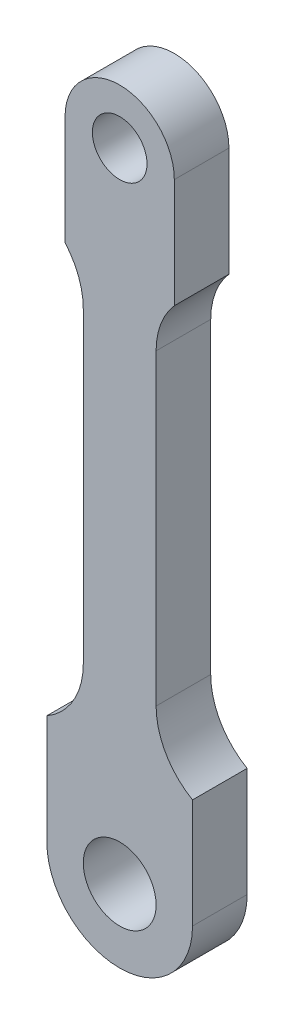
SolidWorks part; units mm, degrees
ref_plane "Front Plane" through (0, 0, 0) normal (0, 0, 1) x (1, 0, 0)
ref_plane "Top Plane" through (0, 0, 0) normal (0, 1, 0) x (1, 0, 0)
ref_plane "Right Plane" through (0, 0, 0) normal (1, 0, 0) x (0, 0, -1)
other "Configuration Table"
sketch "Sketch1" plane through (0, 0, 0) normal (0, 0, 1) x (1, 0, 0)
  line L0 (0, 0) -> (0, 50000) construction
  line L1 (-3, 0) -> (-3, -6)
  line L2 (3, 0) -> (3, -6)
  line L3 (-2, -8.6458) -> (-2, -25.5359)
  line L4 (-4, -35) -> (-4, -29)
  line L5 (4, -35) -> (4, -29)
  line L6 (2, -8.6458) -> (2, -25.5359)
  circle A0 centre (0, 0) radius 1.5
  arc A1 (3, 0) -> (-3, 0) centre (0, 0) ccw
  circle A2 centre (0, -35) radius 2
  arc A3 (-4, -35) -> (4, -35) centre (0, -35) ccw
  arc A4 (-2, -8.6458) -> (-3, -6) centre (-6, -8.6458) ccw
  arc A5 (2, -8.6458) -> (3, -6) centre (6, -8.6458) cw
  arc A6 (-4, -29) -> (-2, -25.5359) centre (-6, -25.5359) ccw
  arc A7 (4, -29) -> (2, -25.5359) centre (6, -25.5359) cw
  dimension "D1" = 3
  dimension "D2" = 6
  dimension "D5" = 4
  dimension "D7" = 8
  dimension "D9" = 8
  dimension "D10" = 8
  dimension "D3" = 6
  dimension "D4" = 4
  dimension "D6" = 35
  dimension "D8" = 6
extrude "Boss-Extrude1" add sketch "Sketch1" along normal mid plane 3
